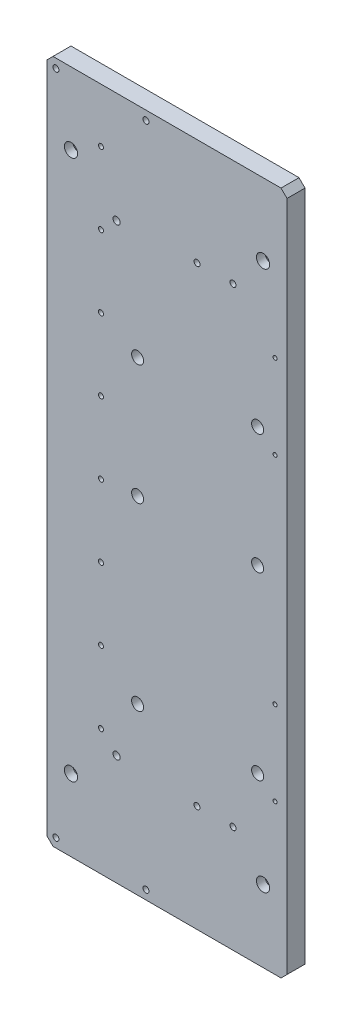
from build123d import *

# Parameters (mm, degrees)
SKETCH_1_W                   = 200
SKETCH_1_H                   = 570
EXTRUDE_1_DEPTH              = 15
CHAMFER_1_SIZE               = 5
MM_0_D                       = 6
HOLE_WIZARD_M6_1_D           = 5
HOLE_WIZARD_M5_2_D           = 4.2
HOLE_WIZARD_M6_2_D           = 5
HOLE_WIZARD_M4_1_D           = 3.3
MM_1_D                       = 1
MM_1_DEPTH                   = 17
MM_1_TIP                     = 0.30043031
HOLE_WIZARD_M5_1_D           = 5.5
HOLE_WIZARD_M5_1_DEPTH       = 17
HOLE_WIZARD_M5_1_CBORE_D     = 10
HOLE_WIZARD_M5_1_CBORE_DEPTH = 7
HOLE_WIZARD_M5_1_TIP         = 1.652366702
HOLE_WIZARD_1_D              = 6.6
HOLE_WIZARD_1_CBORE_D        = 11
HOLE_WIZARD_1_CBORE_DEPTH    = 7


with BuildPart() as part:
    # 草图1 → 凸台-拉伸1 (new body)
    with BuildSketch(Plane.XY):
        Rectangle(SKETCH_1_W, SKETCH_1_H)
    extrude(amount=EXTRUDE_1_DEPTH)

    # 倒角1
    chamfer_1_edges = [part.edges().sort_by_distance(p)[0] for p in [
        (100, -285, 7.5),
        (-100, -285, 7.5),
        (-100, 285, 7.5),
        (100, 285, 7.5),
    ]]
    chamfer(chamfer_1_edges, length=CHAMFER_1_SIZE)

    # 大小mm 暗销孔0 (through all)
    with Locations(Plane.XY.offset(15)):
        with Locations((-42, -193), (258, -193), (-42, 193), (258, 193)):
            Hole(MM_0_D / 2)

    # M6 螺纹孔1 (through all)
    with Locations(Plane.XY.offset(15)):
        with Locations((55, 196), (25, 196), (55, -196), (25, -196)):
            Hole(HOLE_WIZARD_M6_1_D / 2)

    # M5 螺纹孔2 (through all)
    with Locations(Plane.XY.offset(15)):
        with Locations((-55, 240), (-55, 180), (-55, 120), (-55, 60), (-55, 0), (-55, -60), (-55, -120), (-55, -180)):
            Hole(HOLE_WIZARD_M5_2_D / 2)

    # M6 螺纹孔2 (through all)
    with Locations(Plane.XY.offset(15)):
        with Locations((-92.500000001, -277.499999995), (-17.500000001, -277.499999995), (-17.499999995, 277.500000015), (-92.499999995, 277.500000015)):
            Hole(HOLE_WIZARD_M6_2_D / 2)

    # M4 螺纹孔1 (through all)
    with Locations(Plane.XY.offset(15)):
        with Locations((90, -160), (90, -90), (90, 90), (90, 160)):
            Hole(HOLE_WIZARD_M4_1_D / 2)

    # 大小mm 暗销孔1
    with Locations(Plane(origin=(0, 0, 0), x_dir=(-1, 0, 0), z_dir=(0, 0, -1))):
        with Locations((24.5, 103), (-75.5, 103), (24.5, -147), (-75.5, -147), (24.5, 3), (-75.5, 3)):
            Hole(MM_1_D / 2, depth=MM_1_DEPTH)
            with Locations((0, 0, -(MM_1_DEPTH + MM_1_TIP / 2))):  # 118° drill point
                Cone(0, MM_1_D / 2, MM_1_TIP, mode=Mode.SUBTRACT)

    # M5 六角凹头螺钉的柱形沉头孔1
    with Locations(Plane.XY.offset(15)):
        with Locations((75.5, -147), (75.5, 103), (75.5, 3), (-24.5, 103), (-24.5, 3), (-24.5, -147)):
            CounterBoreHole(HOLE_WIZARD_M5_1_D / 2, HOLE_WIZARD_M5_1_CBORE_D / 2, HOLE_WIZARD_M5_1_CBORE_DEPTH, depth=HOLE_WIZARD_M5_1_DEPTH)
            with Locations((0, 0, -(HOLE_WIZARD_M5_1_DEPTH + HOLE_WIZARD_M5_1_TIP / 2))):  # 118° drill point
                Cone(0, HOLE_WIZARD_M5_1_D / 2, HOLE_WIZARD_M5_1_TIP, mode=Mode.SUBTRACT)

    # 打孔尺寸(%根据)内六角花形圆柱头螺钉1 (through all)
    with Locations(Plane.XY.offset(15)):
        with Locations((-80, -225), (80, -225), (-80, 225), (80, 225)):
            CounterBoreHole(HOLE_WIZARD_1_D / 2, HOLE_WIZARD_1_CBORE_D / 2, HOLE_WIZARD_1_CBORE_DEPTH)


solid = part.part
